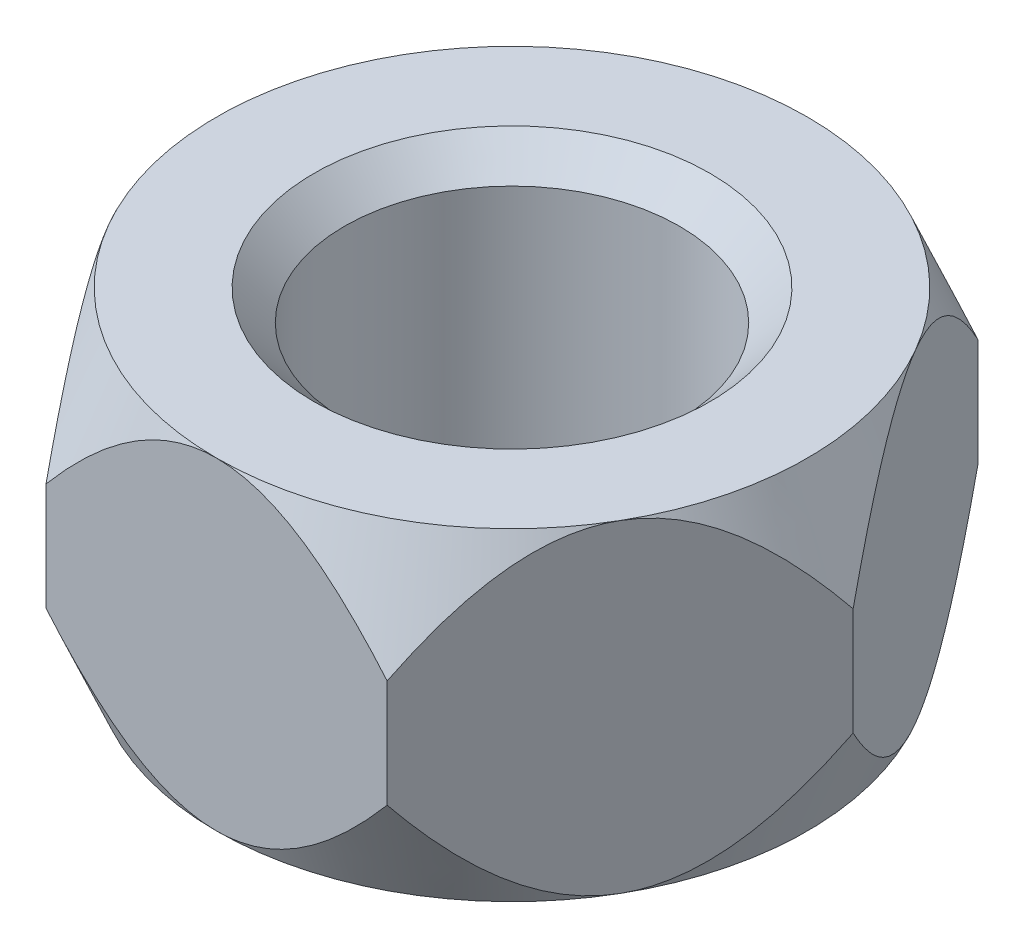
from build123d import *

# Parameters (mm, degrees)
BOSS_EXTRUDE1_DEPTH          = 8.2
SKETCH2_OUTSIDE_W            = 31.148
SKETCH2_OUTSIDE_H            = 28.828
SKETCH2_OUTSIDE_R            = 7.5
CUT_EXTRUDE1_DEPTH           = 8.2
CUT_EXTRUDE1_DRAFT           = -23
SKETCH3_OUTSIDE_W            = 31.148
SKETCH3_OUTSIDE_H            = 28.828
SKETCH3_OUTSIDE_R            = 7.5
CUT_EXTRUDE2_DEPTH           = 8.2
CUT_EXTRUDE2_DRAFT           = -23
M10_TAPPED_HOLE1_D           = 8.5
M10_TAPPED_HOLE1_CSINK_D     = 10.05
M10_TAPPED_HOLE1_CSINK_ANGLE = 90


with BuildPart() as part:
    # Sketch1 → Boss-Extrude1 (new body)
    with BuildSketch(Plane(origin=(0, 0, 0), x_dir=(1, 0, 0), z_dir=(0, 1, 0))):
        Polygon((4.330127019, 7.5), (-4.330127019, 7.5), (-8.660254038, 0), (-4.330127019, -7.5), (4.330127019, -7.5), (8.660254038, 0), align=None)
    extrude(amount=BOSS_EXTRUDE1_DEPTH)


with BuildPart() as cut_extrude1_tool:
    # Sketch2 outside → Cut-Extrude1 (with draft: the straight prism first)
    with BuildSketch(Plane(origin=(0, 8.2, 0), x_dir=(1, 0, 0), z_dir=(0, 1, 0))):
        Rectangle(SKETCH2_OUTSIDE_W, SKETCH2_OUTSIDE_H)
        Circle(SKETCH2_OUTSIDE_R, mode=Mode.SUBTRACT)
    extrude(amount=-CUT_EXTRUDE1_DEPTH)
    # Cut-Extrude1: the draft: its side faces are tilted about the plane it starts from
    cut_extrude1_sides = [cut_extrude1_tool.faces().sort_by_distance(p)[0] for p in [
        (0, 4.1, 14.414),
        (15.574, 4.1, 0),
        (0, 4.1, -14.414),
        (-15.574, 4.1, 0),
        (-7.5, 4.1, 0),
    ]]
    draft(cut_extrude1_sides, Plane(origin=(0, 8.2, 0), x_dir=(1, 0, 0), z_dir=(0, 1, 0)), CUT_EXTRUDE1_DRAFT)


with BuildPart() as part_1:
    add(part.part)

    # Cut-Extrude1: cut by cut_extrude1_tool
    add(cut_extrude1_tool.part, mode=Mode.SUBTRACT)


with BuildPart() as cut_extrude2_tool:
    # Sketch3 outside → Cut-Extrude2 (with draft: the straight prism first)
    with BuildSketch(Plane.XZ):
        Rectangle(SKETCH3_OUTSIDE_W, SKETCH3_OUTSIDE_H)
        Circle(SKETCH3_OUTSIDE_R, mode=Mode.SUBTRACT)
    extrude(amount=-CUT_EXTRUDE2_DEPTH)
    # Cut-Extrude2: the draft: its side faces are tilted about the plane it starts from
    cut_extrude2_sides = [cut_extrude2_tool.faces().sort_by_distance(p)[0] for p in [
        (0, 4.1, -14.414),
        (15.574, 4.1, 0),
        (0, 4.1, 14.414),
        (-15.574, 4.1, 0),
        (-7.5, 4.1, 0),
    ]]
    draft(cut_extrude2_sides, Plane.XZ, CUT_EXTRUDE2_DRAFT)


with BuildPart() as part_2:
    add(part_1.part)

    # Cut-Extrude2: cut by cut_extrude2_tool
    add(cut_extrude2_tool.part, mode=Mode.SUBTRACT)

    # M10 Tapped Hole1 (through all)
    with Locations(Plane(origin=(0, 8.2, 0), x_dir=(1, 0, 0), z_dir=(0, 1, 0))):
        with Locations((0, 0)):
            CounterSinkHole(M10_TAPPED_HOLE1_D / 2, M10_TAPPED_HOLE1_CSINK_D / 2, counter_sink_angle=M10_TAPPED_HOLE1_CSINK_ANGLE)


solid = part_2.part
